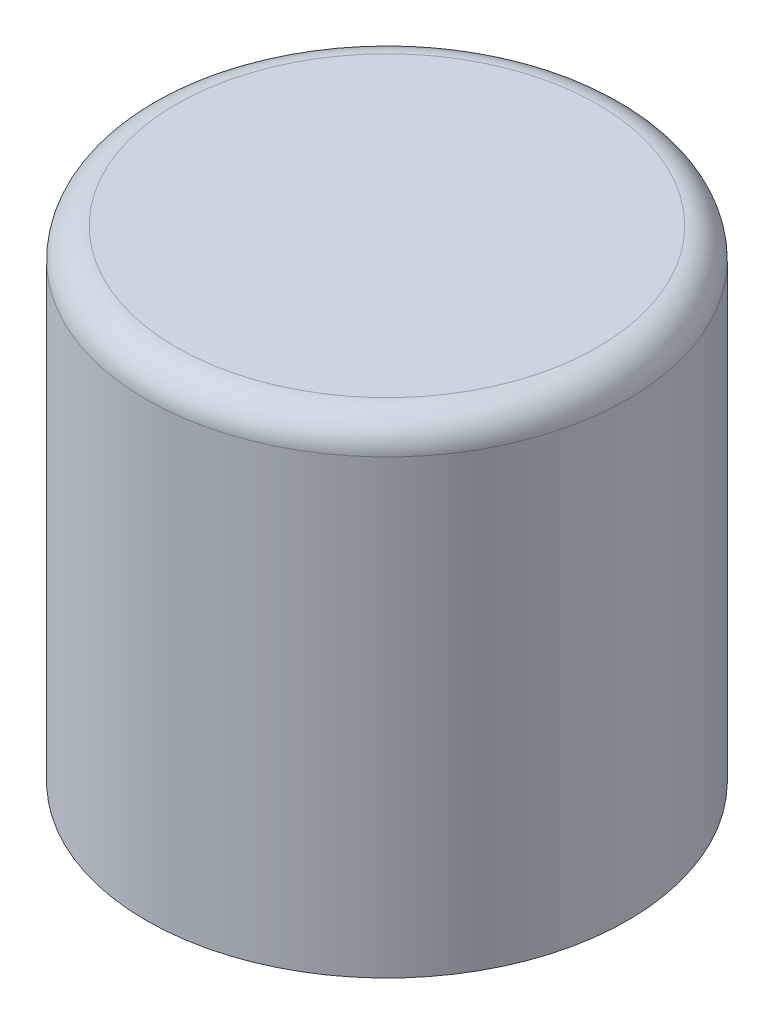
SolidWorks part; units mm, degrees
material "20#"
ref_plane "Front Plane" through (0, 0, 0) normal (0, 0, 1) x (1, 0, 0)
ref_plane "Top Plane" through (0, 0, 0) normal (0, 1, 0) x (1, 0, 0)
ref_plane "Right Plane" through (0, 0, 0) normal (1, 0, 0) x (0, 0, -1)
sketch "Sketch1" plane through (0, 0, 0) normal (0, 1, 0) x (1, 0, 0)
  circle A0 centre (0, 0) radius 40
  dimension "D1" = 80
extrude "Boss-Extrude1" add sketch "Sketch1" along normal blind 80
fillet "Fillet1" radius 5 1 edges at (0, 80, 40)
